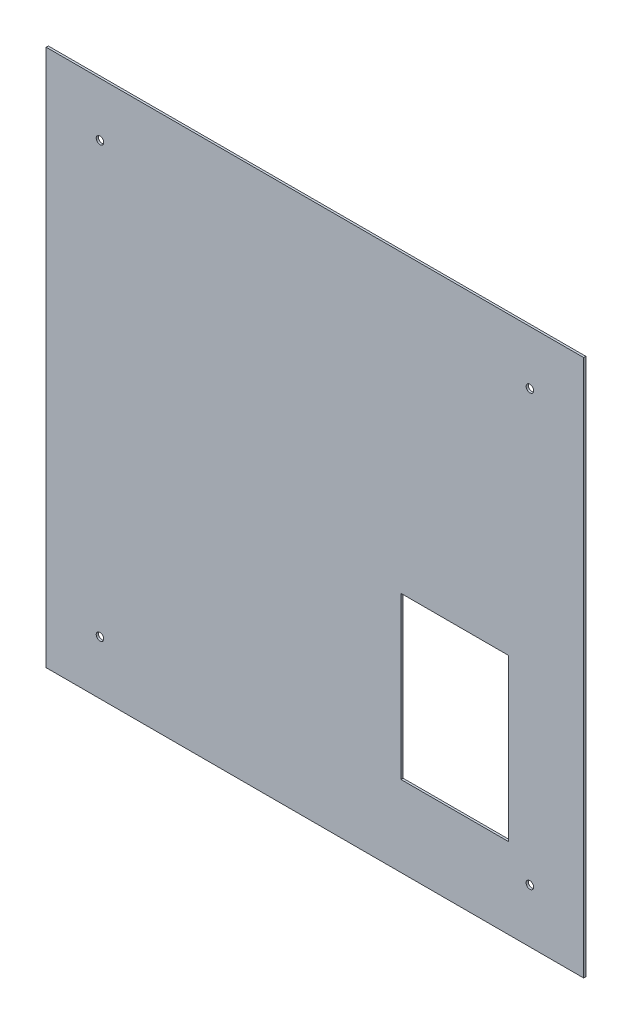
SolidWorks part; units mm, degrees
ref_plane "前视基准面" through (0, 0, 0) normal (0, 0, 1) x (1, 0, 0)
ref_plane "上视基准面" through (0, 0, 0) normal (0, 1, 0) x (1, 0, 0)
ref_plane "右视基准面" through (0, 0, 0) normal (1, 0, 0) x (0, 0, -1)
sketch "草图1" plane through (0, 0, 0) normal (0, 0, 1) x (1, 0, 0)
  line L1 (-250, 250) -> (250, 250)
  line L2 (-250, 250) -> (-250, -250)
  line L3 (-250, -250) -> (250, -250)
  line L4 (250, 250) -> (250, -250)
  line L5 (-250, 250) -> (250, -250) construction
  line L6 (-250, -250) -> (250, 250) construction
  point P0 (0, 0)
  dimension "D1" = 500
  dimension "D2" = 500
extrude "凸台-拉伸1" add sketch "草图1" along normal blind 2
hole_wizard "Ø7.0 (7) 直径孔1" positions "草图2" profile "草图3" hole size "Ø7.0" standard "GB" end condition through all
sketch "草图2" plane through (0, 0, 2) normal (0, 0, 1) x (1, 0, 0)
  line L0 (0, 392.1954) -> (0, 0) construction
  line L1 (0, 0) -> (378.3177, 0) construction
  point P0 (-200, 200)
  point P2 (200, 200)
  point P4 (-200, -200)
  point P6 (200, -200)
  dimension "D1" = 400
  dimension "D2" = 400
sketch "草图3" plane through (-200, 200, 2) normal (1, 0, 0) x (0, -1, 0)
  line L0 (0, 0) -> (0, 2)
  line L1 (0, 2) -> (3.5, 2)
  line L2 (3.5, 2) -> (3.5, 0)
  line L5 (3.5, 0) -> (0, 0)
  line L11 (0, -6.35) -> (0, 107.95) construction
  dimension "通孔孔直径" = 7
  dimension "通孔孔深度" = 2
sketch "草图4" plane through (0, 0, 2) normal (0, 0, 1) x (1, 0, 0)
  line L0 (250, 250) -> (-250, 250) construction
  line L1 (80, -25) -> (180, -25)
  line L2 (80, -25) -> (80, -175)
  line L3 (80, -175) -> (180, -175)
  line L4 (180, -25) -> (180, -175)
  line L5 (80, -25) -> (180, -175) construction
  line L6 (80, -175) -> (180, -25) construction
  line L7 (-250, 250) -> (-250, -250) construction
  point P0 (130, -100)
  dimension "D1" = 275
  dimension "D2" = 330
  dimension "D3" = 100
  dimension "D4" = 150
extrude "切除-拉伸1" cut sketch "草图4" against normal through all
